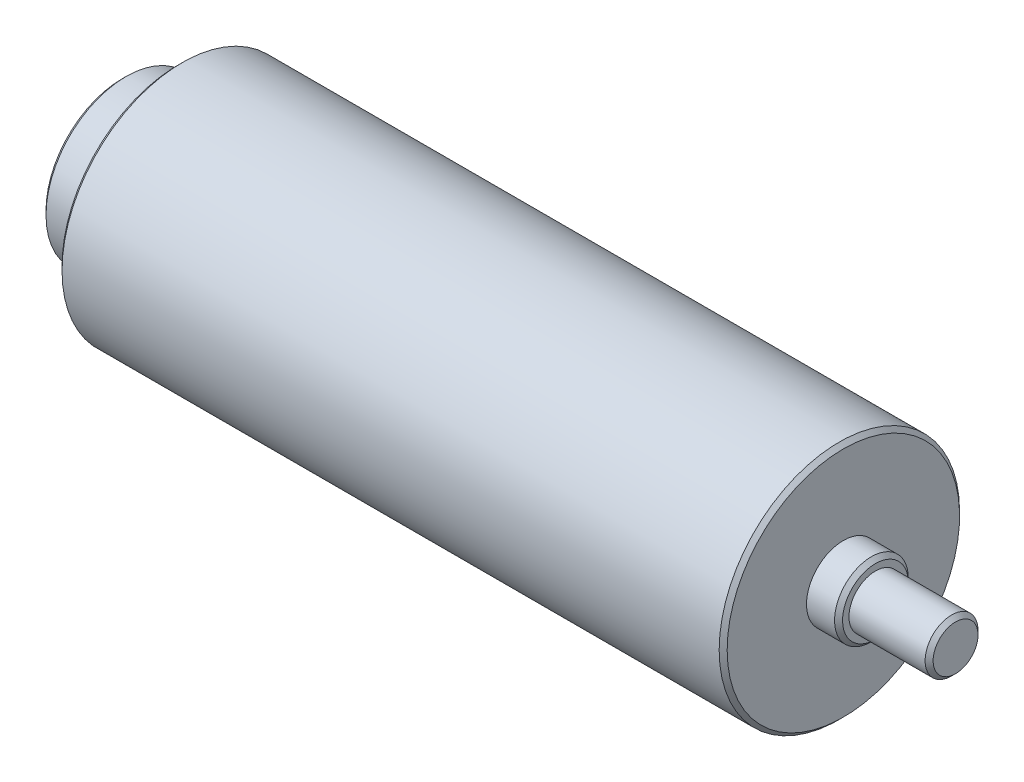
SolidWorks part; units mm, degrees
material "Q235B"
ref_plane "Front Plane" through (0, 0, 0) normal (0, 0, 1) x (1, 0, 0)
ref_plane "Top Plane" through (0, 0, 0) normal (0, 1, 0) x (1, 0, 0)
ref_plane "Right Plane" through (0, 0, 0) normal (1, 0, 0) x (0, 0, -1)
sketch "Sketch1" plane through (0, 0, 0) normal (0, 0, 1) x (1, 0, 0)
  line L0 (695.5088, 30.6496) -> (685.5088, 30.6496)
  line L2 (685.5088, 30.6496) -> (685.5088, 31.9496)
  line L5 (681.5088, 31.9496) -> (681.5088, 42.3496)
  line L6 (681.5088, 42.3496) -> (598.5088, 42.3496)
  line L7 (598.5088, -275) -> (598.5088, 225) construction
  line L8 (700.5088, 27.3496) -> (682.5088, 27.3496) construction
  line L9 (700.5088, 21.8648) -> (700.5088, 32.8344) construction
  line L10 (682.5088, -155.2055) -> (682.5088, 155.8496) construction
  line L11 (695.5088, 30.6496) -> (695.5088, 27.3496)
  line L12 (690.5088, -155.2055) -> (690.5088, 155.8496) construction
  line L13 (598.5088, 42.3496) -> (598.5088, 37.3496)
  line L14 (598.5088, 37.3496) -> (591.5088, 37.3496)
  line L15 (591.5088, 37.3496) -> (591.5088, 27.3496)
  line L16 (682.5088, 27.3496) -> (590.5088, 27.3496) construction
  line L17 (590.5088, -275) -> (590.5088, 225) construction
  line L18 (695.5088, 27.3496) -> (591.5088, 27.3496)
  line L19 (685.5088, 31.9496) -> (681.5088, 31.9496)
  dimension "D1" = 1
  dimension "D2" = 4
  dimension "D3" = 5
  dimension "D4" = 30
  dimension "D5" = 20
  dimension "D6" = 7
  dimension "D7" = 6.6
  dimension "D8" = 9.2
revolve "Revolve1" add sketch "Sketch1" angle 360 about L18
chamfer "Chamfer1" distance 0.5 angle 45 5 edges at (591.5088, 37.3496, 0) (598.5088, 42.3496, 0) (681.5088, 42.3496, 0) (685.5088, 31.9496, 0) (695.5088, 30.6496, 0)
